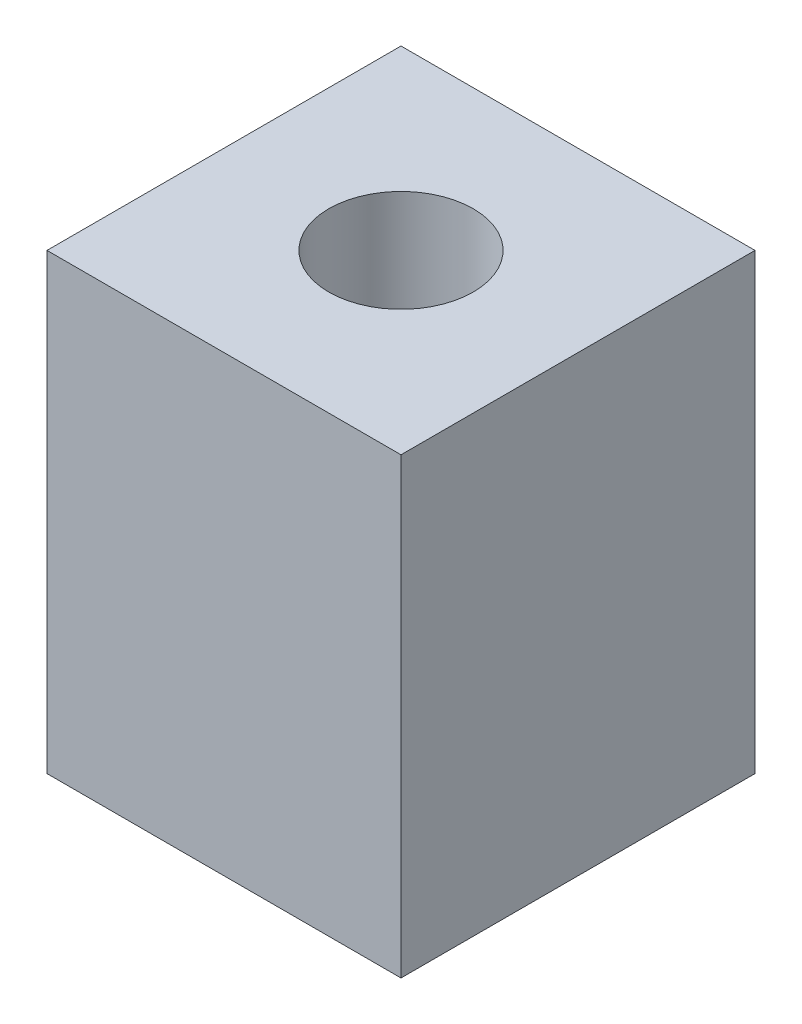
SolidWorks part; units mm, degrees
material "SS400B"
ref_plane "Front Plane" through (0, 0, 0) normal (0, 0, 1) x (1, 0, 0)
ref_plane "Top Plane" through (0, 0, 0) normal (0, 1, 0) x (1, 0, 0)
ref_plane "Right Plane" through (0, 0, 0) normal (1, 0, 0) x (0, 0, -1)
sketch "Sketch1" plane through (0, 0, 0) normal (0, 1, 0) x (1, 0, 0)
  line L1 (-12.5, 12.5) -> (12.5, 12.5)
  line L2 (-12.5, 12.5) -> (-12.5, -12.5)
  line L3 (-12.5, -12.5) -> (12.5, -12.5)
  line L4 (12.5, 12.5) -> (12.5, -12.5)
  line L5 (-12.5, 12.5) -> (12.5, -12.5) construction
  line L6 (-12.5, -12.5) -> (12.5, 12.5) construction
  point P0 (0, 0)
  dimension "D1" = 25
  dimension "D2" = 25
extrude "Boss-Extrude1" add sketch "Sketch1" along normal blind 32
hole_wizard "M12 Tapped Hole1" positions "Sketch2" profile "Sketch3" tap size "M12" standard "GB" end condition through all
sketch "Sketch2" plane through (0, 32, 0) normal (0, 1, 0) x (1, 0, 0)
  point P0 (0, 0)
cosmetic thread "Tapped hole thread1" parameters "D2"=12
sketch "Sketch3" plane through (0, 32, 0) normal (1, 0, 0) x (0, 0, 1)
  line L0 (0, 0) -> (0, 32)
  line L1 (0, 32) -> (5.1, 32)
  line L2 (5.1, 32) -> (5.1, 0)
  line L5 (5.1, 0) -> (0, 0)
  line L11 (0, -6.35) -> (0, 107.95) construction
  dimension "通孔螺纹孔钻头直径" = 10.2
  dimension "通孔螺纹孔钻头深度" = 32
